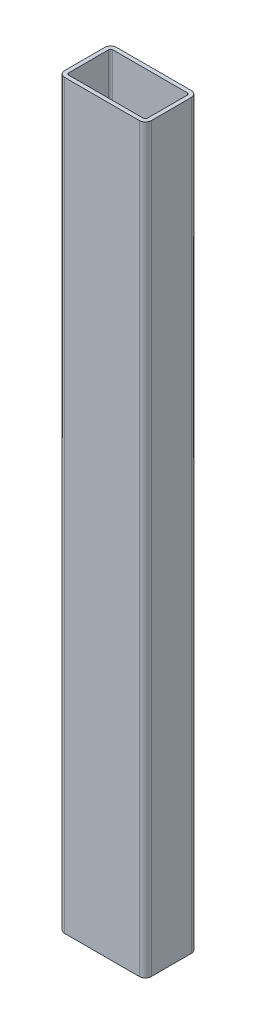
from build123d import *

# Parameters (mm, degrees)
BOSS_EXTRUDE1_DEPTH = 428


with BuildPart() as part:
    # Sketch1 → Boss-Extrude1 (new body)
    with BuildSketch(Plane(origin=(0, 0, 0), x_dir=(1, 0, 0), z_dir=(0, 1, 0))):
        with BuildLine():
            Line((-21.55, -15), (21.55, -15))
            ThreePointArc((21.55, -15), (23.989518395, -13.989518395), (25, -11.55))
            Line((25, -11.55), (25, 11.55))
            ThreePointArc((25, 11.55), (23.989518395, 13.989518395), (21.55, 15))
            Line((21.55, 15), (-21.55, 15))
            ThreePointArc((-21.55, 15), (-23.989518395, 13.989518395), (-25, 11.55))
            Line((-25, 11.55), (-25, -11.55))
            ThreePointArc((-25, -11.55), (-23.989518395, -13.989518395), (-21.55, -15))
        make_face()
        with BuildLine():
            Line((-21.55, -12.7), (21.55, -12.7))
            ThreePointArc((21.55, -12.7), (22.363172798, -12.363172798), (22.7, -11.55))
            Line((22.7, -11.55), (22.7, 11.55))
            ThreePointArc((22.7, 11.55), (22.363172798, 12.363172798), (21.55, 12.7))
            Line((21.55, 12.7), (-21.55, 12.7))
            ThreePointArc((-21.55, 12.7), (-22.363172798, 12.363172798), (-22.7, 11.55))
            Line((-22.7, 11.55), (-22.7, -11.55))
            ThreePointArc((-22.7, -11.55), (-22.363172798, -12.363172798), (-21.55, -12.7))
        make_face(mode=Mode.SUBTRACT)
    extrude(amount=BOSS_EXTRUDE1_DEPTH)


solid = part.part
